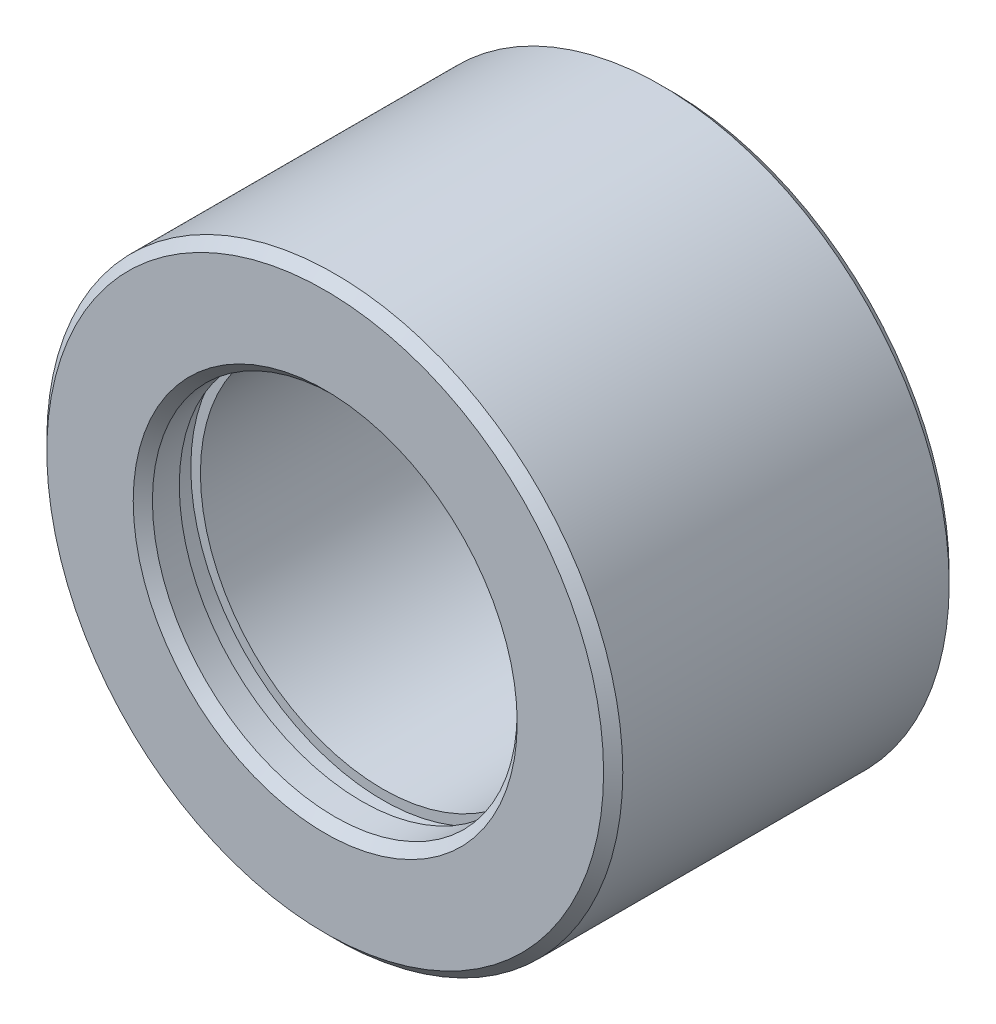
from build123d import *

# Parameters (mm, degrees)
SKETCH1_R           = 15
SKETCH1_R_2         = 9.5
BOSS_EXTRUDE1_DEPTH = 9
CUT_EXTRUDE1_START  = 6
SKETCH2_R           = 10
SKETCH2_R_2         = 9.5
CUT_EXTRUDE1_DEPTH  = 1.1
CHAMFER1_SIZE       = 0.5


with BuildPart() as part:
    # Sketch1 → Boss-Extrude1 (new, symmetric)
    with BuildSketch(Plane.XY):
        Circle(SKETCH1_R)
        Circle(SKETCH1_R_2, mode=Mode.SUBTRACT)
    extrude(amount=BOSS_EXTRUDE1_DEPTH, both=True)

    # Sketch2 → Cut-Extrude1 (cut)
    with BuildSketch(Plane.XY.offset(CUT_EXTRUDE1_START)):
        Circle(SKETCH2_R)
        Circle(SKETCH2_R_2, mode=Mode.SUBTRACT)
    cut_extrude1 = extrude(amount=CUT_EXTRUDE1_DEPTH, mode=Mode.SUBTRACT)

    # Mirror1: Cut-Extrude1 across plane
    add(cut_extrude1.mirror(Plane.XY), mode=Mode.SUBTRACT)

    # Chamfer1
    chamfer1_edges = [part.edges().sort_by_distance(p)[0] for p in [
        (-15, 0, -9),
        (-15, 0, 9),
        (-9.5, 0, -9),
        (-9.5, 0, 9),
    ]]
    chamfer(chamfer1_edges, length=CHAMFER1_SIZE)


solid = part.part
